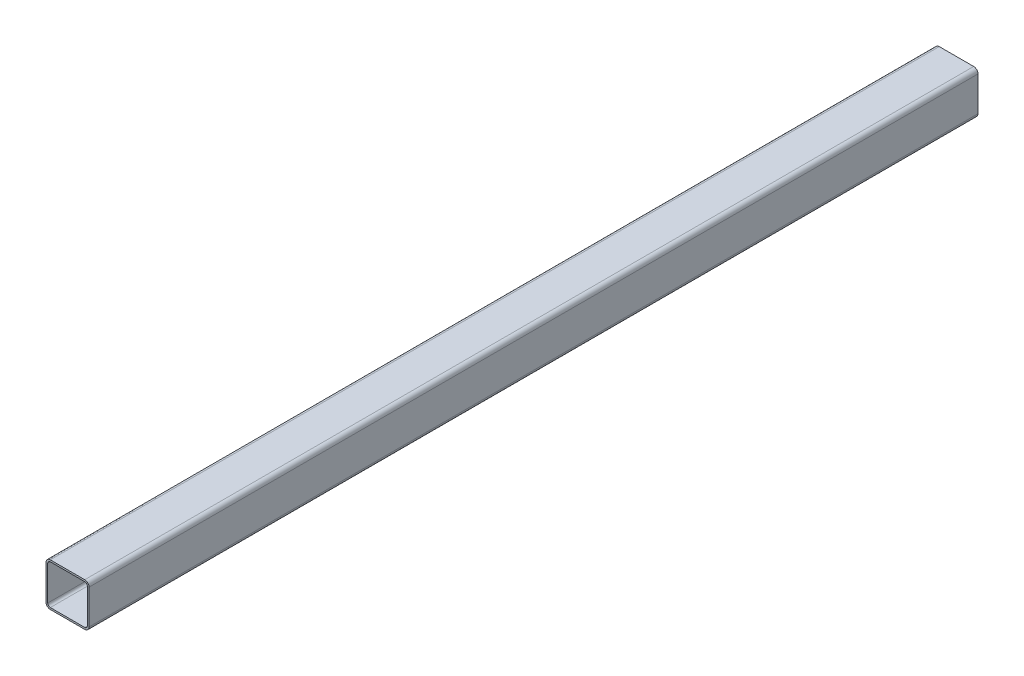
from build123d import *

# Parameters (mm, degrees)
BOSS_EXTRUDE1_DEPTH = 4130


with BuildPart() as part:
    # Sketch1 → Boss-Extrude1 (new body)
    with BuildSketch(Plane.XY):
        with BuildLine():
            Line((-80, 100), (80, 100))
            ThreePointArc((80, 100), (94.142135624, 94.142135624), (100, 80))
            Line((100, 80), (100, -80))
            ThreePointArc((100, -80), (94.142135624, -94.142135624), (80, -100))
            Line((80, -100), (-80, -100))
            ThreePointArc((-80, -100), (-94.142135624, -94.142135624), (-100, -80))
            Line((-100, -80), (-100, 80))
            ThreePointArc((-100, 80), (-94.142135624, 94.142135624), (-80, 100))
        make_face()
        with BuildLine():
            Line((-92, 80), (-92, -80))
            ThreePointArc((-92, -80), (-88.485281374, -88.485281374), (-80, -92))
            Line((-80, -92), (80, -92))
            ThreePointArc((80, -92), (88.485281374, -88.485281374), (92, -80))
            Line((92, -80), (92, 80))
            ThreePointArc((92, 80), (88.485281374, 88.485281374), (80, 92))
            Line((80, 92), (-80, 92))
            ThreePointArc((-80, 92), (-88.485281374, 88.485281374), (-92, 80))
        make_face(mode=Mode.SUBTRACT)
    extrude(amount=BOSS_EXTRUDE1_DEPTH)


solid = part.part
